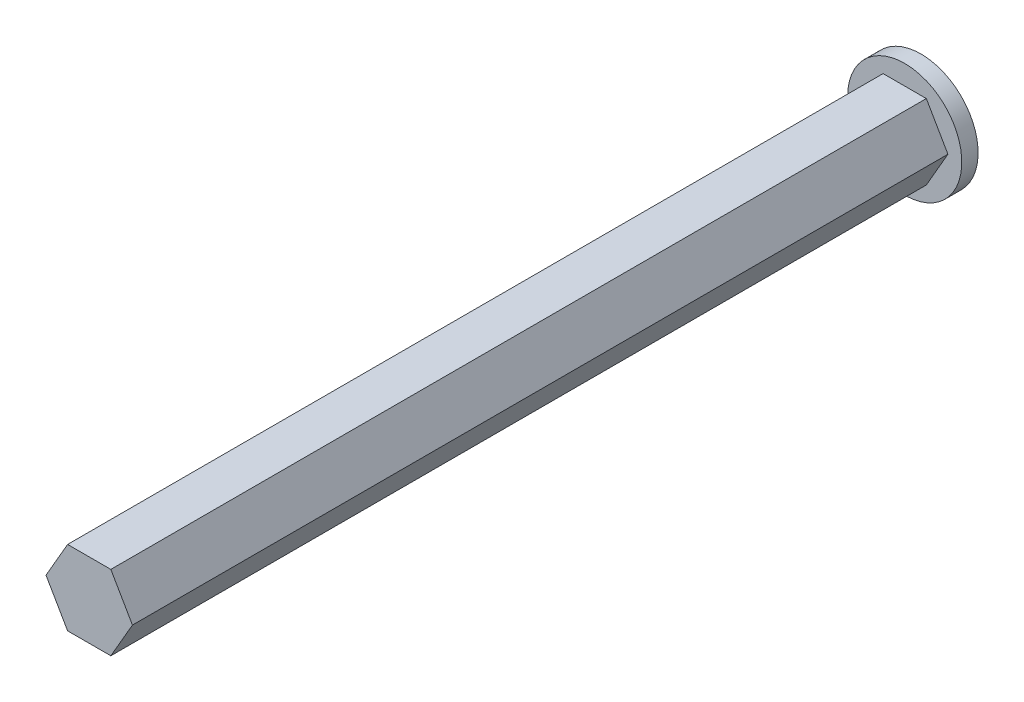
from build123d import *

# Parameters (mm, degrees)
BOSS_EXTRUDE1_DEPTH = 100
SKETCH2_R           = 7
BOSS_EXTRUDE2_DEPTH = 3
CHAMFER1_SIZE       = 1
CHAMFER1_SIZE2      = 1.732050808


with BuildPart() as part:
    # Sketch1 → Boss-Extrude1 (new body)
    with BuildSketch(Plane.XY):
        Polygon((2.65, -4.58993464), (5.3, 0), (2.65, 4.58993464), (-2.65, 4.58993464), (-5.3, 0), (-2.65, -4.58993464), align=None)
    extrude(amount=BOSS_EXTRUDE1_DEPTH)

    # Sketch2 → Boss-Extrude2 (add)
    with BuildSketch(Plane(origin=(0, 0, 0), x_dir=(-1, 0, 0), z_dir=(0, 0, -1))):
        Circle(SKETCH2_R)
    extrude(amount=BOSS_EXTRUDE2_DEPTH)

    # Chamfer1
    chamfer1_edges = [part.edges().sort_by_distance(p)[0] for p in [
        (7, 0, -3),
    ]]
    chamfer1_side = [part.faces().sort_by_distance(p)[0] for p in [
        (7, 0, -1.5),
    ]]
    chamfer(chamfer1_edges, length=CHAMFER1_SIZE, length2=CHAMFER1_SIZE2, reference=chamfer1_side[0])


solid = part.part
